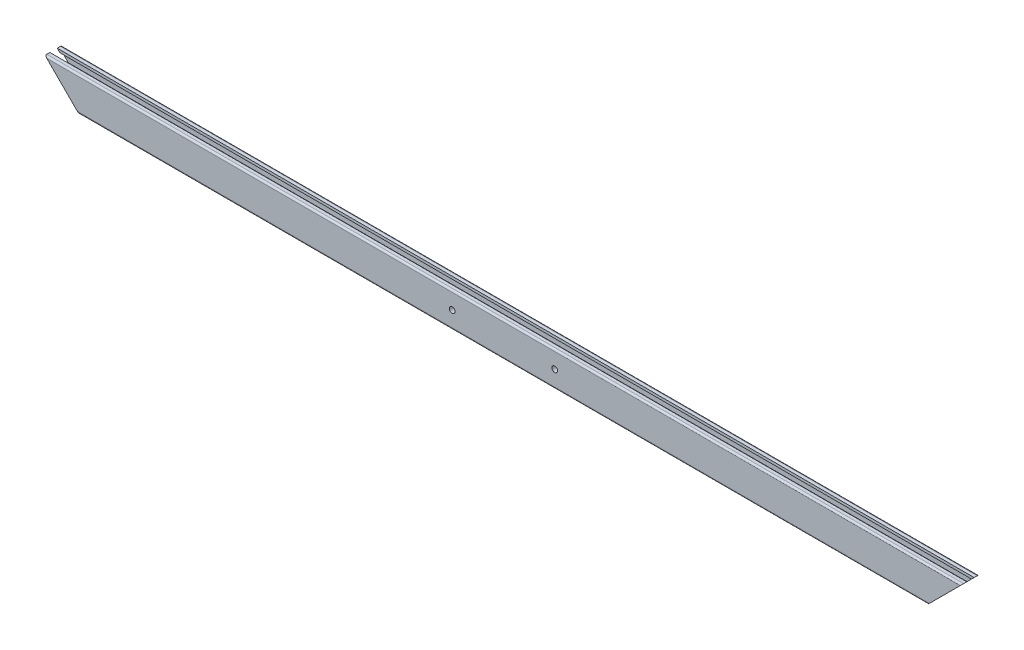
from build123d import *

# Parameters (mm, degrees)
SKETCH11_R          = 2.5
MEMBER_1_DEPTH      = 805
CUT_EXTRUDE_1_DEPTH = 404.058618566
HOLE_WIZARD_M6_1_D  = 5


with BuildPart() as part:
    # Sketch11 → Member 1 (new body)
    with BuildSketch(Plane(origin=(-402.5, 0, 0), x_dir=(0, 0, -1), z_dir=(1, 0, 0))):
        with BuildLine():
            Line((-6, -15), (-3.25, -15))
            Line((-3.25, -15), (-3.25, -12.7))
            Line((-3.25, -12.7), (-5, -12.7))
            Line((-5, -12.7), (-5, -7))
            ThreePointArc((-5, -7), (0, -4.31662479), (5, -7))
            Line((5, -7), (5, -12.7))
            Line((5, -12.7), (3.25, -12.7))
            Line((3.25, -12.7), (3.25, -15))
            Line((3.25, -15), (6, -15))
            ThreePointArc((6, -15), (7.060660172, -14.560660172), (7.5, -13.5))
            Line((7.5, -13.5), (7.5, 13.5))
            ThreePointArc((7.5, 13.5), (7.060660172, 14.560660172), (6, 15))
            Line((6, 15), (3.25, 15))
            Line((3.25, 15), (3.25, 12.7))
            Line((3.25, 12.7), (5, 12.7))
            Line((5, 12.7), (5, 7))
            ThreePointArc((5, 7), (0, 4.31662479), (-5, 7))
            Line((-5, 7), (-5, 12.7))
            Line((-5, 12.7), (-3.25, 12.7))
            Line((-3.25, 12.7), (-3.25, 15))
            Line((-3.25, 15), (-6, 15))
            ThreePointArc((-6, 15), (-7.060660172, 14.560660172), (-7.5, 13.5))
            Line((-7.5, 13.5), (-7.5, -13.5))
            ThreePointArc((-7.5, -13.5), (-7.060660172, -14.560660172), (-6, -15))
        make_face()
        Circle(SKETCH11_R, mode=Mode.SUBTRACT)
    extrude(amount=MEMBER_1_DEPTH)

    # 草图4 → 切除-拉伸1 (cut, through all)
    with BuildSketch(Plane.XY.offset(7.5)):
        Polygon((-402.5, 15), (-372.5, -15), (-402.5, -15), align=None)
        Polygon((402.5, -15), (402.5, 15), (372.5, -15), align=None)
    extrude(amount=-CUT_EXTRUDE_1_DEPTH, mode=Mode.SUBTRACT)

    # M6 螺纹孔1 (through all)
    with Locations(Plane.XY.offset(7.5)):
        with Locations((-45, 0), (45, 0)):
            Hole(HOLE_WIZARD_M6_1_D / 2)


solid = part.part
